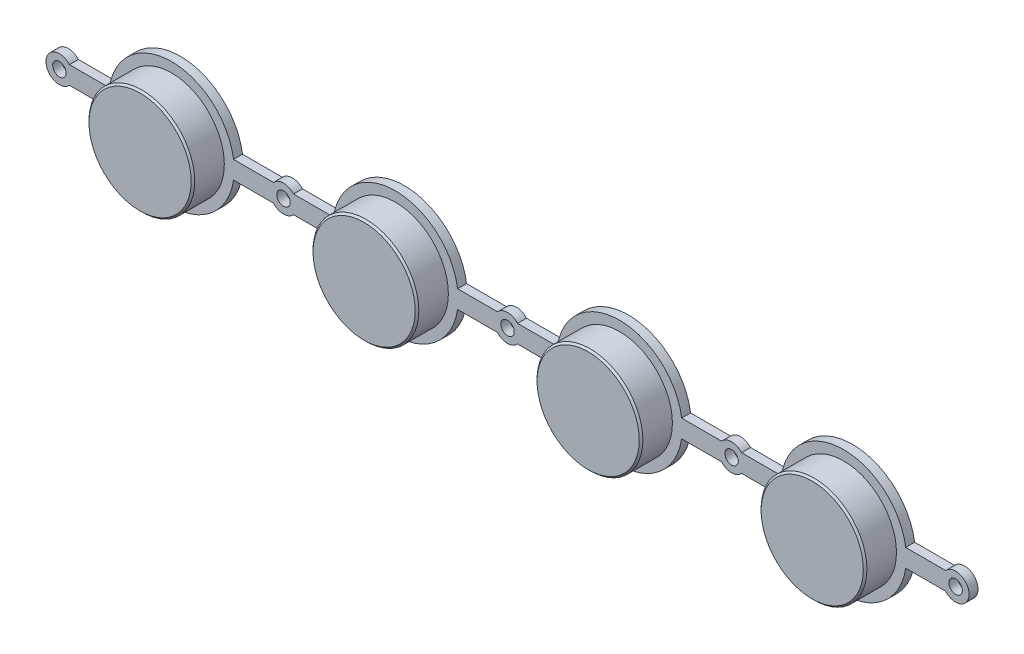
SolidWorks part; units mm, degrees
ref_plane "Front Plane" through (0, 0, 0) normal (0, 0, 1) x (1, 0, 0)
ref_plane "Top Plane" through (0, 0, 0) normal (0, 1, 0) x (1, 0, 0)
ref_plane "Right Plane" through (0, 0, 0) normal (1, 0, 0) x (0, 0, -1)
other "Configuration Table"
sketch "Sketch1" plane through (0, 0, 0) normal (0, 0, 1) x (1, 0, 0)
  line L0 (0, 0) -> (75, 0) construction
  line L1 (0, 0) -> (-12.5, 0) construction
  line L2 (75, 0) -> (87.5, 0) construction
  line L3 (-11.382, 1) -> (-6.9282, 1)
  line L4 (-11.382, -1) -> (-6.9282, -1)
  line L5 (6.9282, -1) -> (11.382, -1)
  line L6 (6.9282, 1) -> (11.382, 1)
  line L7 (13.618, 1) -> (18.0718, 1)
  line L8 (13.618, -1) -> (18.0718, -1)
  line L9 (31.9282, -1) -> (36.382, -1)
  line L10 (31.9282, 1) -> (36.382, 1)
  line L11 (38.618, 1) -> (43.0718, 1)
  line L12 (38.618, -1) -> (43.0718, -1)
  line L13 (56.9282, -1) -> (61.382, -1)
  line L14 (56.9282, 1) -> (61.382, 1)
  line L15 (63.618, 1) -> (68.0718, 1)
  line L16 (63.618, -1) -> (68.0718, -1)
  line L17 (81.9282, 1) -> (86.382, 1)
  line L18 (81.9282, -1) -> (86.382, -1)
  arc A4 (-6.9282, -1) -> (6.9282, -1) centre (0, 0) ccw
  arc A5 (18.0718, -1) -> (31.9282, -1) centre (25, 0) ccw
  arc A6 (43.0718, -1) -> (56.9282, -1) centre (50, 0) ccw
  arc A7 (68.0718, -1) -> (81.9282, -1) centre (75, 0) ccw
  circle A8 centre (12.5, 0) radius 0.75
  circle A9 centre (37.5, 0) radius 0.75
  circle A10 centre (62.5, 0) radius 0.75
  arc A11 (11.382, -1) -> (13.618, -1) centre (12.5, 0) ccw
  arc A12 (36.382, -1) -> (38.618, -1) centre (37.5, 0) ccw
  arc A13 (61.382, -1) -> (63.618, -1) centre (62.5, 0) ccw
  circle A14 centre (-12.5, 0) radius 0.75
  arc A15 (-11.382, 1) -> (-11.382, -1) centre (-12.5, 0) ccw
  circle A16 centre (87.5, 0) radius 0.75
  arc A17 (86.382, -1) -> (86.382, 1) centre (87.5, 0) ccw
  arc A18 (6.9282, 1) -> (-6.9282, 1) centre (0, 0) ccw
  arc A19 (13.618, 1) -> (11.382, 1) centre (12.5, 0) ccw
  arc A20 (31.9282, 1) -> (18.0718, 1) centre (25, 0) ccw
  arc A21 (38.618, 1) -> (36.382, 1) centre (37.5, 0) ccw
  arc A22 (56.9282, 1) -> (43.0718, 1) centre (50, 0) ccw
  arc A23 (63.618, 1) -> (61.382, 1) centre (62.5, 0) ccw
  arc A24 (81.9282, 1) -> (68.0718, 1) centre (75, 0) ccw
  dimension "D2" = 14
  dimension "D3" = 25
  dimension "D4" = 25
  dimension "D5" = 1.5
  dimension "D6" = 3
  dimension "D7" = 12.5
  dimension "D8" = 12.5
  dimension "D1" = 75
  dimension "D9" = 12.5
  dimension "D10" = 12.5
  dimension "D11" = 2
extrude "Boss-Extrude1" add sketch "Sketch1" along normal blind 1
sketch "Sketch2" plane through (0, 0, 1) normal (0, 0, 1) x (1, 0, 0)
  circle A0 centre (0, 0) radius 5.9
  circle A1 centre (25, 0) radius 5.9
  circle A2 centre (50, 0) radius 5.9
  circle A3 centre (75, 0) radius 5.9
  dimension "D1" = 11.8
extrude "Boss-Extrude2" add sketch "Sketch2" along normal blind 3.5
chamfer "Chamfer1" distance 0.2 angle 45 4 edges at (80.9, 0, 4.5) (55.9, 0, 4.5) (30.9, 0, 4.5) (5.9, 0, 4.5)
sketch "Sketch3" plane through (0, 0, 0) normal (0, 0, -1) x (-1, 0, 0)
  line L0 (-74.25, -0.75) -> (-74.25, -4)
  line L1 (-75.75, 4) -> (-74.25, 4)
  line L2 (-75.75, 4) -> (-75.75, 0.75)
  line L3 (-75.75, -4) -> (-74.25, -4)
  line L4 (-74.25, 4) -> (-74.25, 0.75)
  line L5 (-75.75, 4) -> (-74.25, -4) construction
  line L6 (-75.75, -4) -> (-74.25, 4) construction
  line L7 (-79, 0.75) -> (-75.75, 0.75)
  line L8 (-79, 0.75) -> (-79, -0.75)
  line L9 (-79, -0.75) -> (-75.75, -0.75)
  line L10 (-71, 0.75) -> (-71, -0.75)
  line L11 (-79, 0.75) -> (-71, -0.75) construction
  line L12 (-79, -0.75) -> (-71, 0.75) construction
  line L13 (-50.75, 4) -> (-49.25, 4)
  line L14 (-50.75, 4) -> (-50.75, 0.75)
  line L15 (-50.75, -4) -> (-49.25, -4)
  line L16 (-49.25, 4) -> (-49.25, 0.75)
  line L17 (-50.75, 4) -> (-49.25, -4) construction
  line L18 (-50.75, -4) -> (-49.25, 4) construction
  line L19 (-54, 0.75) -> (-50.75, 0.75)
  line L20 (-54, 0.75) -> (-54, -0.75)
  line L21 (-54, -0.75) -> (-50.75, -0.75)
  line L22 (-46, 0.75) -> (-46, -0.75)
  line L23 (-54, 0.75) -> (-46, -0.75) construction
  line L24 (-54, -0.75) -> (-46, 0.75) construction
  line L25 (-29, 0.75) -> (-25.75, 0.75)
  line L26 (-29, 0.75) -> (-29, -0.75)
  line L27 (-29, -0.75) -> (-25.75, -0.75)
  line L28 (-21, 0.75) -> (-21, -0.75)
  line L29 (-29, 0.75) -> (-21, -0.75) construction
  line L30 (-29, -0.75) -> (-21, 0.75) construction
  line L31 (-25.75, 4) -> (-24.25, 4)
  line L32 (-25.75, 4) -> (-25.75, 0.75)
  line L33 (-25.75, -4) -> (-24.25, -4)
  line L34 (-24.25, 4) -> (-24.25, 0.75)
  line L35 (-25.75, 4) -> (-24.25, -4) construction
  line L36 (-25.75, -4) -> (-24.25, 4) construction
  line L37 (-4, 0.75) -> (-0.75, 0.75)
  line L38 (-4, 0.75) -> (-4, -0.75)
  line L39 (-4, -0.75) -> (-0.75, -0.75)
  line L40 (4, 0.75) -> (4, -0.75)
  line L41 (-4, 0.75) -> (4, -0.75) construction
  line L42 (-4, -0.75) -> (4, 0.75) construction
  line L43 (-0.75, 4) -> (0.75, 4)
  line L44 (-0.75, 4) -> (-0.75, 0.75)
  line L45 (-0.75, -4) -> (0.75, -4)
  line L46 (0.75, 4) -> (0.75, 0.75)
  line L47 (-0.75, 4) -> (0.75, -4) construction
  line L48 (-0.75, -4) -> (0.75, 4) construction
  line L49 (-74.25, -0.75) -> (-71, -0.75)
  line L51 (-75.75, -0.75) -> (-75.75, -4)
  line L54 (-74.25, 0.75) -> (-71, 0.75)
  line L58 (-49.25, 0.75) -> (-46, 0.75)
  line L60 (-49.25, -0.75) -> (-49.25, -4)
  line L61 (-49.25, -0.75) -> (-46, -0.75)
  line L63 (-50.75, -0.75) -> (-50.75, -4)
  line L65 (-25.75, -0.75) -> (-25.75, -4)
  line L68 (-24.25, 0.75) -> (-21, 0.75)
  line L70 (-24.25, -0.75) -> (-24.25, -4)
  line L71 (-24.25, -0.75) -> (-21, -0.75)
  line L73 (0.75, 0.75) -> (4, 0.75)
  line L76 (-0.75, -0.75) -> (-0.75, -4)
  line L78 (0.75, -0.75) -> (0.75, -4)
  line L79 (0.75, -0.75) -> (4, -0.75)
  point P0 (-75, 0)
  point P6 (-75, 0)
  point P11 (-50, 0)
  point P17 (-50, 0)
  point P22 (-25, 0)
  point P28 (-25, 0)
  point P33 (0, 0)
  point P39 (0, 0)
  dimension "D1" = 8
  dimension "D2" = 8
  dimension "D3" = 1.5
  dimension "D4" = 1.5
  dimension "D5" = 8
  dimension "D6" = 8
  dimension "D7" = 1.5
  dimension "D8" = 1.5
  dimension "D9" = 8
  dimension "D10" = 8
  dimension "D11" = 1.5
  dimension "D12" = 1.5
  dimension "D13" = 8
  dimension "D14" = 8
  dimension "D15" = 1.5
  dimension "D16" = 1.5
extrude "Boss-Extrude3" add sketch "Sketch3" along normal blind 2
chamfer "Chamfer2" distance 1.6 angle 45 16 edges at (-4, 0, -2) (0, -4, -2) (0, 4, -2) (4, 0, -2) (25, 4, -2) (21, 0, -2) (29, 0, -2) (25, -4, -2) (50, 4, -2) (46, 0, -2) (50, -4, -2) (54, 0, -2) (75, 4, -2) (79, 0, -2) (71, 0, -2) (75, -4, -2)
